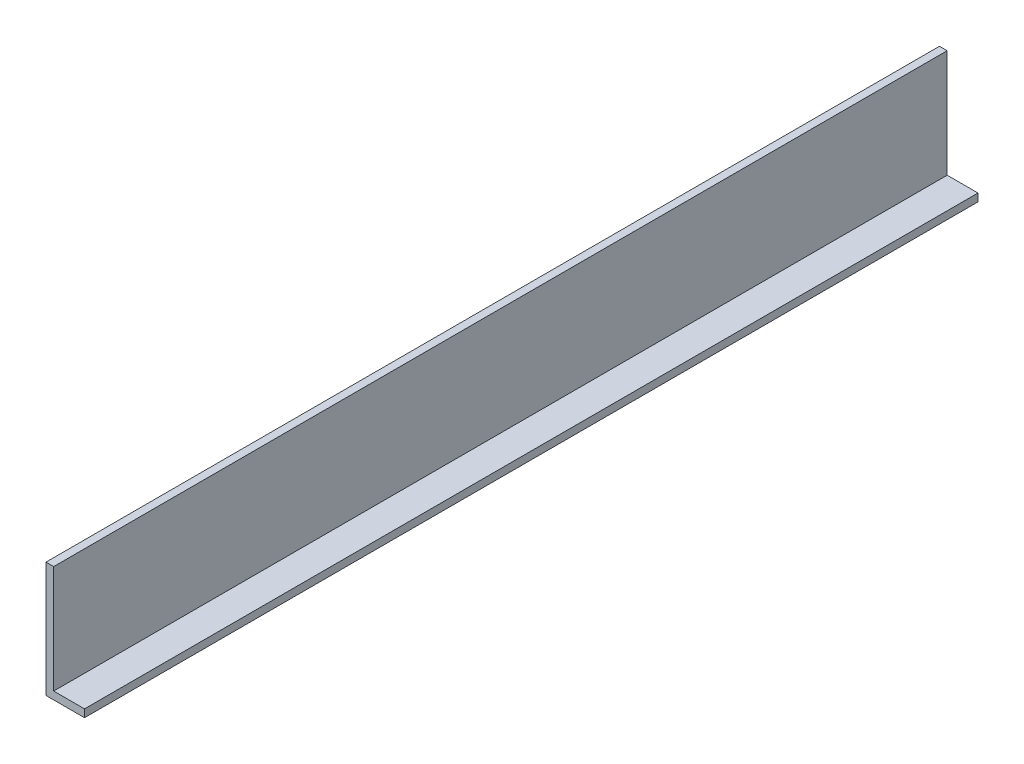
from build123d import *

# Parameters (mm, degrees)
EXTRUDE_1_DEPTH = 116


with BuildPart() as part:
    # 草图1 → 拉伸-薄壁1 (new, symmetric)
    with BuildSketch(Plane.XY):
        Polygon((10, 0), (0, 0), (0, 30), (2, 30), (2, 2), (10, 2), align=None)
    extrude(amount=EXTRUDE_1_DEPTH, both=True)


solid = part.part
